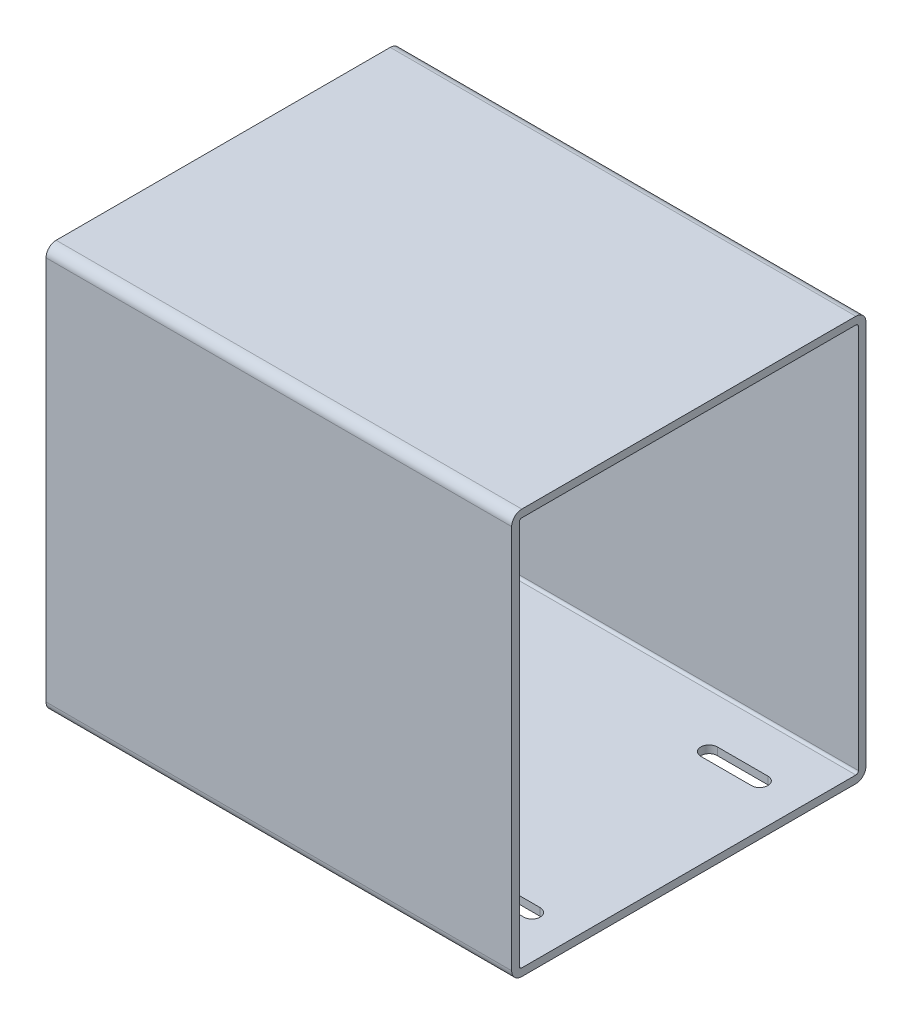
from build123d import *

# Parameters (mm, degrees)
EXTRUDE_1_DEPTH      = 150
EXTRUDE_1_DEPTH_BACK = 34
SKETCH_2_W           = 140
SKETCH_2_H           = 160
SKETCH_2_W_2         = 134
SKETCH_2_H_2         = 154
CUT_EXTRUDE_1_DEPTH  = 10
FILLET_1_R           = 1
FILLET_2_R           = 4


with BuildPart() as part:
    # 草图2 → 凸台-拉伸1 (new, two sides: drawn at the far end of the back side and taken through both)
    with BuildSketch(Plane(origin=(0, 0, 0), x_dir=(0, 0, -1), z_dir=(1, 0, 0)).offset(-EXTRUDE_1_DEPTH_BACK)):
        Rectangle(SKETCH_2_W, SKETCH_2_H)
        Rectangle(SKETCH_2_W_2, SKETCH_2_H_2, mode=Mode.SUBTRACT)
    extrude(amount=EXTRUDE_1_DEPTH + EXTRUDE_1_DEPTH_BACK)

    # 草图3 → 切除-拉伸1 (cut)
    with BuildSketch(Plane(origin=(0, -77, 0), x_dir=(1, 0, 0), z_dir=(0, 1, 0))):
        with BuildLine():
            Line((-17, 48.25), (3, 48.25))
            ThreePointArc((3, 48.25), (6.25, 45), (3, 41.75))
            Line((3, 41.75), (-17, 41.75))
            ThreePointArc((-17, 41.75), (-20.25, 45), (-17, 48.25))
        make_face()
        with BuildLine():
            Line((-17, -48.25), (3, -48.25))
            ThreePointArc((3, -48.25), (6.25, -45), (3, -41.75))
            Line((3, -41.75), (-17, -41.75))
            ThreePointArc((-17, -41.75), (-20.25, -45), (-17, -48.25))
        make_face()
        with BuildLine():
            Line((133, 48.25), (113, 48.25))
            ThreePointArc((113, 48.25), (109.75, 45), (113, 41.75))
            Line((113, 41.75), (133, 41.75))
            ThreePointArc((133, 41.75), (136.25, 45), (133, 48.25))
        make_face()
        with BuildLine():
            Line((133, -48.25), (113, -48.25))
            ThreePointArc((113, -48.25), (109.75, -45), (113, -41.75))
            Line((113, -41.75), (133, -41.75))
            ThreePointArc((133, -41.75), (136.25, -45), (133, -48.25))
        make_face()
    extrude(amount=-CUT_EXTRUDE_1_DEPTH, mode=Mode.SUBTRACT)

    # 圆角1
    fillet_1_edges = [part.edges().sort_by_distance(p)[0] for p in [
        (58, -77, 67),
        (58, 77, 67),
        (58, 77, -67),
        (58, -77, -67),
    ]]
    fillet(fillet_1_edges, radius=FILLET_1_R)

    # 圆角2
    fillet_2_edges = [part.edges().sort_by_distance(p)[0] for p in [
        (58, -80, -70),
        (58, -80, 70),
        (58, 80, 70),
        (58, 80, -70),
    ]]
    fillet(fillet_2_edges, radius=FILLET_2_R)


solid = part.part
